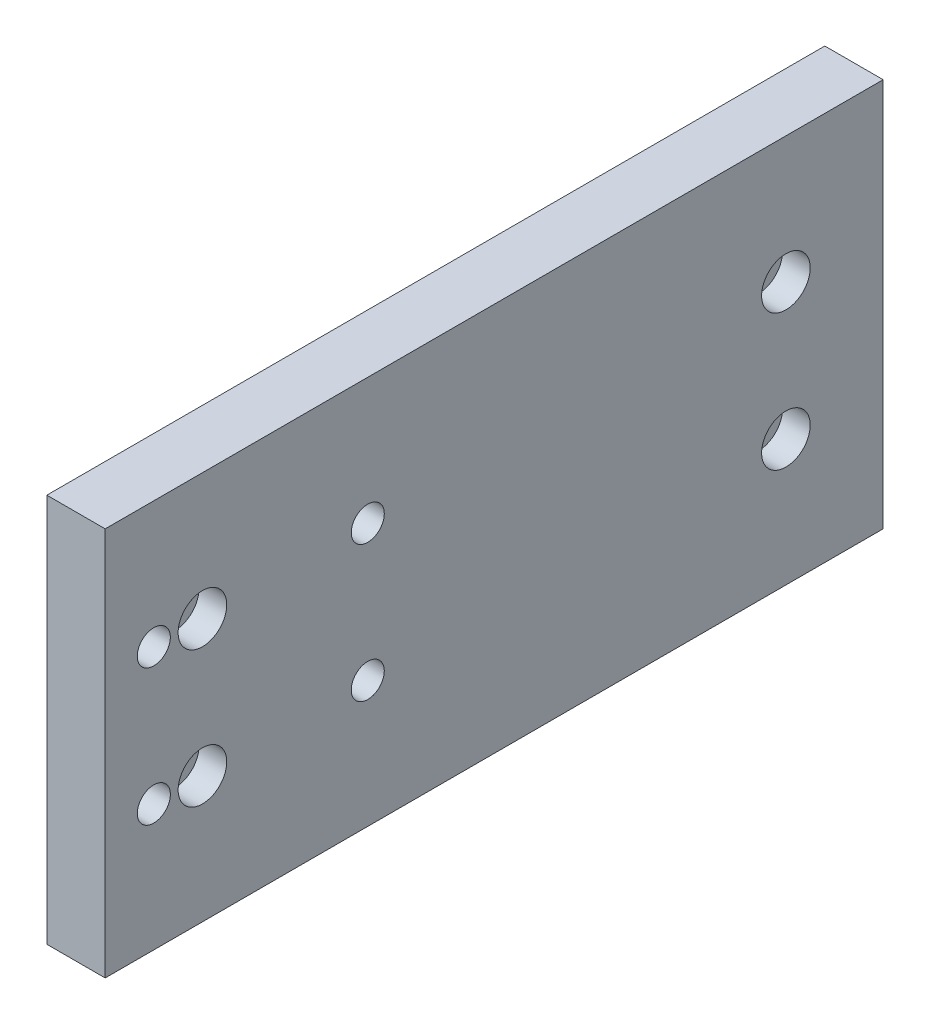
SolidWorks part; units mm, degrees
ref_plane "前视基准面" through (0, 0, 0) normal (0, 0, 1) x (1, 0, 0)
ref_plane "上视基准面" through (0, 0, 0) normal (0, 1, 0) x (1, 0, 0)
ref_plane "右视基准面" through (0, 0, 0) normal (1, 0, 0) x (0, 0, -1)
sketch "草图1" plane through (0, 0, 0) normal (1, 0, 0) x (0, 0, -1)
  line L1 (-80, 40) -> (80, 40)
  line L2 (-80, 40) -> (-80, -40)
  line L3 (-80, -40) -> (80, -40)
  line L4 (80, 40) -> (80, -40)
  line L5 (-80, 40) -> (80, -40) construction
  line L6 (-80, -40) -> (80, 40) construction
  point P0 (0, 0)
  dimension "D1" = 160
  dimension "D2" = 80
extrude "凸台-拉伸1" add sketch "草图1" along normal blind 12
hole_wizard "M8 螺纹孔1" positions "草图2" profile "草图3" tap size "M8" standard "GB" end condition through all
sketch "草图2" plane through (12, 0, 0) normal (1, 0, 0) x (0, 0, -1)
  line L0 (-48, 62.2251) -> (-48, 0) construction
  line L1 (-48, 0) -> (70.822, 0) construction
  line L2 (-80, 40) -> (-80, -40) construction
  point P0 (-70, 14)
  point P2 (-70, -14)
  point P4 (-26, 14)
  point P6 (-26, -14)
  dimension "D1" = 44
  dimension "D2" = 28
  dimension "D3" = 10
sketch "草图3" plane through (12, 14, 70) normal (0, 1, 0) x (0, 0, -1)
  line L0 (0, 0) -> (0, 12)
  line L1 (0, 12) -> (3.4, 12)
  line L2 (3.4, 12) -> (3.4, 0)
  line L5 (3.4, 0) -> (0, 0)
  line L11 (0, -6.35) -> (0, 107.95) construction
  dimension "通孔螺纹孔钻头直径" = 6.8
  dimension "通孔螺纹孔钻头深度" = 12
cosmetic thread "孔螺蚊线1" parameters "D2"=8
cosmetic thread "孔螺蚊线2" parameters "D2"=8
cosmetic thread "孔螺蚊线3" parameters "D2"=8
cosmetic thread "孔螺蚊线4" parameters "D2"=8
hole_wizard "打孔尺寸(%根据)内六角圆柱头螺钉的类型1" positions "草图4" profile "草图5" counterbore size "M5" standard "GB" end condition through all
sketch "草图4" plane through (12, 0, 0) normal (1, 0, 0) x (0, 0, -1)
  line L0 (-80, 0) -> (45.8295, 0) construction
  line L1 (-80, 40) -> (-80, -40) construction
  point P0 (-60, 14)
  point P2 (-60, -14)
  point P4 (60, 14)
  point P6 (60, -14)
  dimension "D1" = 120
  dimension "D2" = 28
  dimension "D3" = 20
sketch "草图5" plane through (12, 14, 60) normal (0, 1, 0) x (0, 0, -1)
  line L0 (0, 0) -> (0, 12)
  line L1 (0, 12) -> (2.75, 12)
  line L3 (2.75, 12) -> (2.75, 5.7)
  line L4 (2.75, 5.7) -> (5, 5.7)
  line L5 (5, 5.7) -> (5, 0)
  line L7 (5, 0) -> (0, 0)
  line L11 (0, -6.35) -> (0, 107.95) construction
  dimension "通孔孔直径" = 5.5
  dimension "通孔孔深度" = 12
  dimension "柱形沉头孔直径" = 10
  dimension "柱形沉头孔深度" = 5.7
